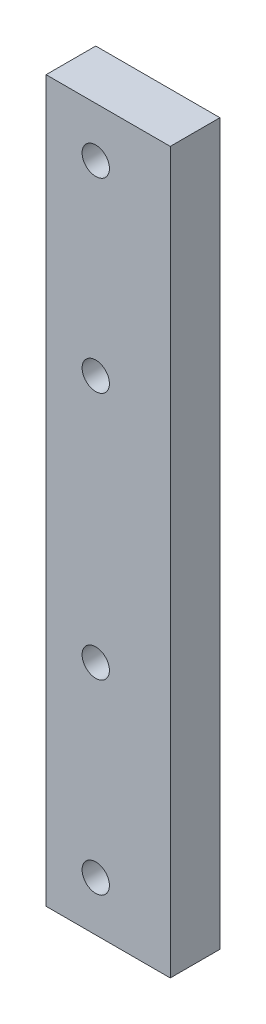
from build123d import *

# Parameters (mm, degrees)
SKETCH_1_W                  = 50
SKETCH_1_H                  = 290
EXTRUDE_1_DEPTH             = 20
HOLE_WIZARD_11_0_11_1_D     = 11
HOLE_WIZARD_11_0_11_1_DEPTH = 36
HOLE_WIZARD_11_0_11_1_TIP   = 3.304733405


with BuildPart() as part:
    # 草图1 → 凸台-拉伸1 (new body)
    with BuildSketch(Plane.XY):
        Rectangle(SKETCH_1_W, SKETCH_1_H)
    extrude(amount=EXTRUDE_1_DEPTH)

    # Ø11.0 (11) 直径孔1
    with Locations(Plane.XY.offset(20)):
        with Locations((-5, 125), (-5, 50), (-5, -50), (-5, -125)):
            Hole(HOLE_WIZARD_11_0_11_1_D / 2, depth=HOLE_WIZARD_11_0_11_1_DEPTH)
            with Locations((0, 0, -(HOLE_WIZARD_11_0_11_1_DEPTH + HOLE_WIZARD_11_0_11_1_TIP / 2))):  # 118° drill point
                Cone(0, HOLE_WIZARD_11_0_11_1_D / 2, HOLE_WIZARD_11_0_11_1_TIP, mode=Mode.SUBTRACT)


solid = part.part
